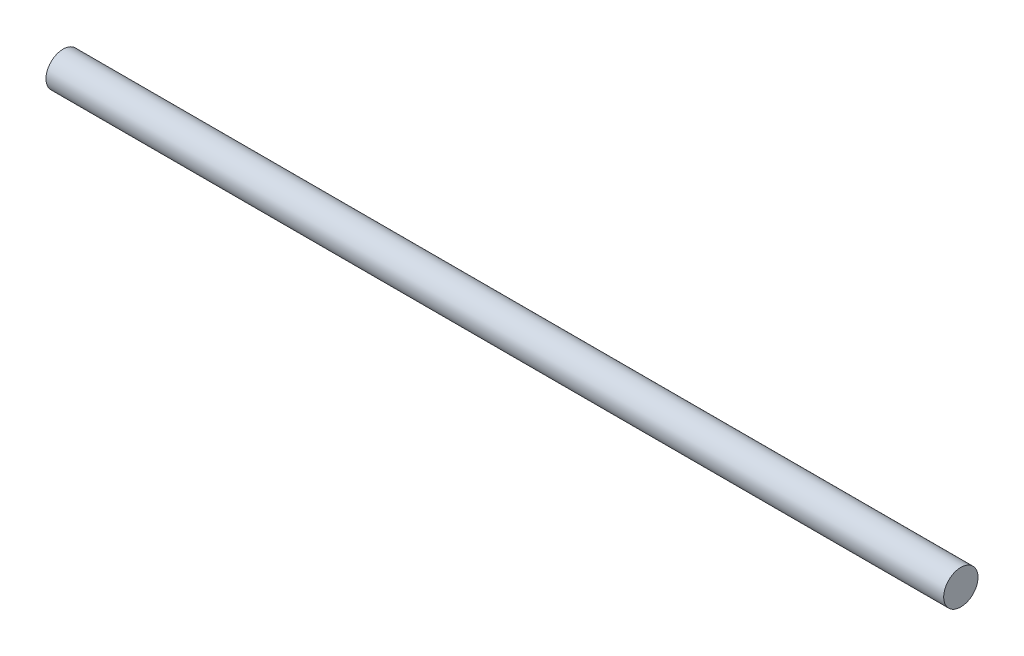
SolidWorks part; units mm, degrees
ref_plane "Front Plane" through (0, 0, 0) normal (0, 0, 1) x (1, 0, 0)
ref_plane "Top Plane" through (0, 0, 0) normal (0, 1, 0) x (1, 0, 0)
ref_plane "Right Plane" through (0, 0, 0) normal (1, 0, 0) x (0, 0, -1)
sketch "Sketch1" plane through (0, 0, 0) normal (1, 0, 0) x (0, 0, -1)
  circle A0 centre (0, 0) radius 6.5
  dimension "D1" = 13
extrude "Boss-Extrude1" add sketch "Sketch1" along normal mid plane 340
